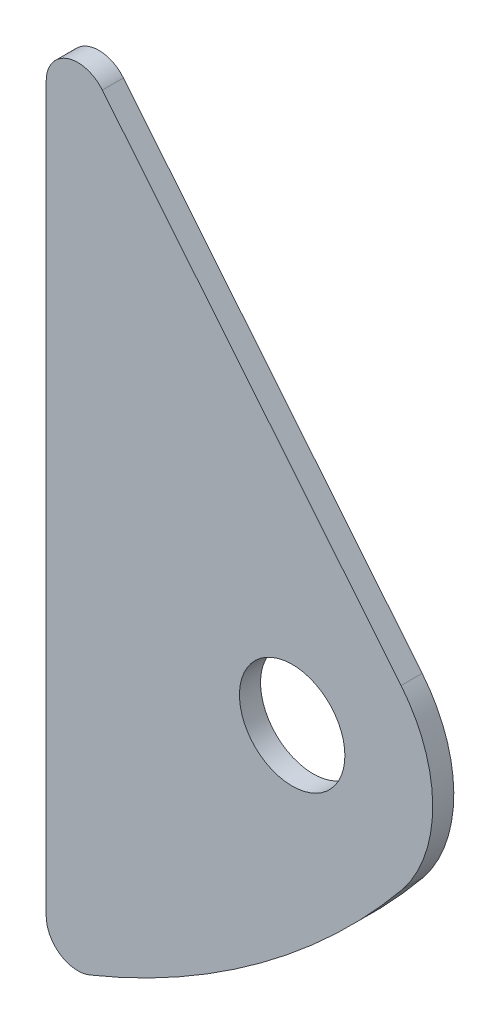
from build123d import *

# Parameters (mm, degrees)
SKETCH1_R           = 30
BOSS_EXTRUDE1_DEPTH = 12


with BuildPart() as part:
    # Sketch1 → Boss-Extrude1 (new body)
    with BuildSketch(Plane.XY):
        with BuildLine():
            Line((-140, 247.683496575), (-140, -164.068744093))
            ThreePointArc((-140, -164.068744093), (-132.043654713, -179.006113339), (-115.208333333, -180.738275097))
            ThreePointArc((-115.208333333, -180.738275097), (-17.836743976, -126.110196806), (63.088864614, -49.191413496))
            ThreePointArc((63.088864614, -49.191413496), (79.995195531, 0.876750818), (61.995559096, 50.562344213))
            Line((61.995559096, 50.562344213), (-108.050999203, 259.060024023))
            ThreePointArc((-108.050999203, 259.060024023), (-128.038128256, 264.640530725), (-140, 247.683496575))
        make_face()
        Circle(SKETCH1_R, mode=Mode.SUBTRACT)
    extrude(amount=BOSS_EXTRUDE1_DEPTH)


solid = part.part
